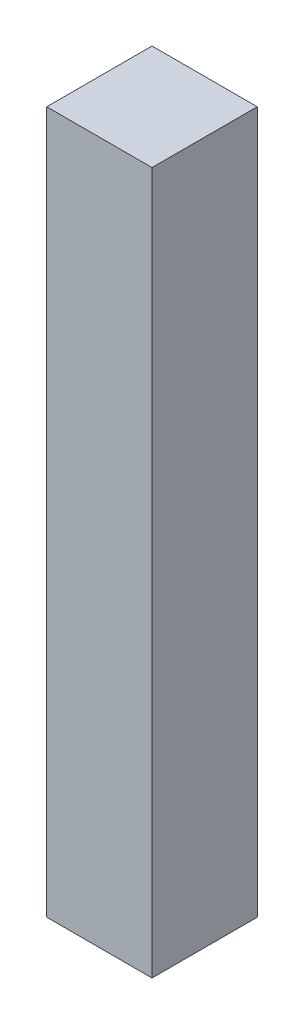
SolidWorks part; units mm, degrees
ref_plane "Front Plane" through (0, 0, 0) normal (0, 0, 1) x (1, 0, 0)
ref_plane "Top Plane" through (0, 0, 0) normal (0, 1, 0) x (1, 0, 0)
ref_plane "Right Plane" through (0, 0, 0) normal (1, 0, 0) x (0, 0, -1)
sketch "Sketch1" plane through (0, 0, 0) normal (0, 1, 0) x (1, 0, 0)
  line L1 (-1.5, -1.5) -> (1.5, -1.5)
  line L2 (-1.5, -1.5) -> (-1.5, 1.5)
  line L3 (-1.5, 1.5) -> (1.5, 1.5)
  line L4 (1.5, -1.5) -> (1.5, 1.5)
  line L5 (-1.5, -1.5) -> (1.5, 1.5) construction
  line L6 (-1.5, 1.5) -> (1.5, -1.5) construction
  point P0 (0, 0)
  dimension "D1" = 3
  dimension "D2" = 3
extrude "Boss-Extrude1" add sketch "Sketch1" along normal blind 20
sketch "Sketch3" plane through (0, 0, 0) normal (0, -1, 0) x (1, 0, 0)
  point P0 (0, 0)
sketch "Sketch4" plane through (0, 20, 0) normal (0, 1, 0) x (1, 0, 0)
  point P0 (0, 0)
